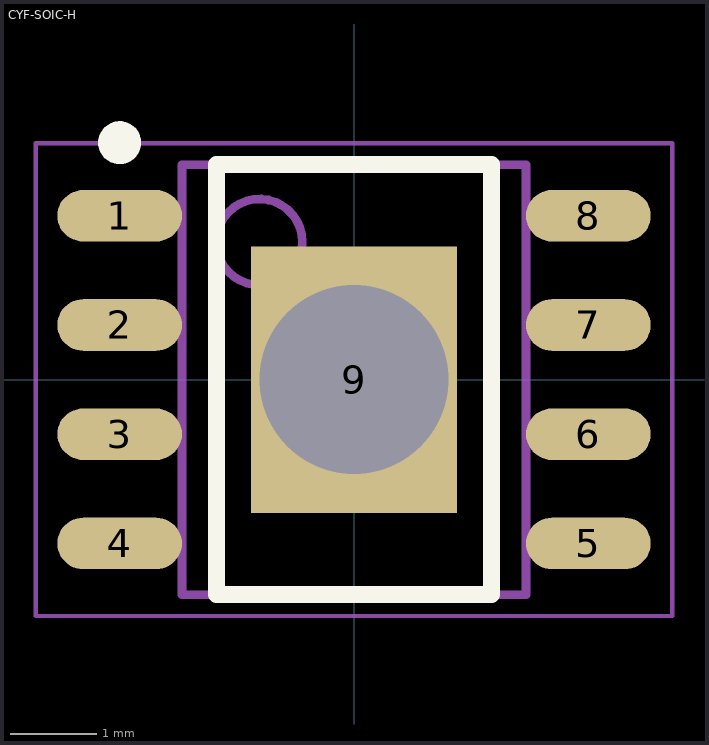
[diagram p0: the footprint, top view; thin cyan lines are the x and y axes]
# Altium footprint library MISC82341.PcbLib: 1 footprints
Each footprint in its own frame and in the unit in brackets; x right, y up, seen from the top. Pads: shape width x height; smd on the part's side, far side on the other; paste and mask are expansions set on the pad; w line width, h text height; cw(c..) or ccw(c..) is an arc to the next point about the centre after c.

## CYF-SOIC-H [mm] "SOIC, 8-Leads, Body 4.90x3.90mm, Pitch 1.27mm, Thermal Pad 3.10x2.40mm, IPC Medium Density"
height 1.7
pads (9):
  oval 1.45x0.6 smd: 1(-2.725,1.905) 2(-2.725,0.635) 3(-2.725,-0.635) 4(-2.725,-1.905) 5(2.725,-1.905) 6(2.725,-0.635) 7(2.725,0.635) 8(2.725,1.905)
  rect 2.4x3.1 hole 2.2: 9(0,0)
Top Overlay:
  circle w0.25: c-2.725,2.755 r0.125
  lines w0.2: -1.6,-2.5 1.6,-2.5 1.6,2.5 -1.6,2.5 -1.6,-2.5
Mechanical 13:
  circle w0.1: c-1.1,1.6 r0.5
  lines w0.1: -2,-2.5 2,-2.5 2,2.5 -2,2.5 -2,-2.5
Mechanical 15:
  lines w0.05: -3.7,-2.75 3.7,-2.75 3.7,2.75 -3.7,2.75 -3.7,-2.75
  lines w0.1: -0.5,0 0.5,0 ; 0,-0.5 0,0.5
3D body: height 1.7, standoff 0.15, extent -2,-2.5 2,2.5